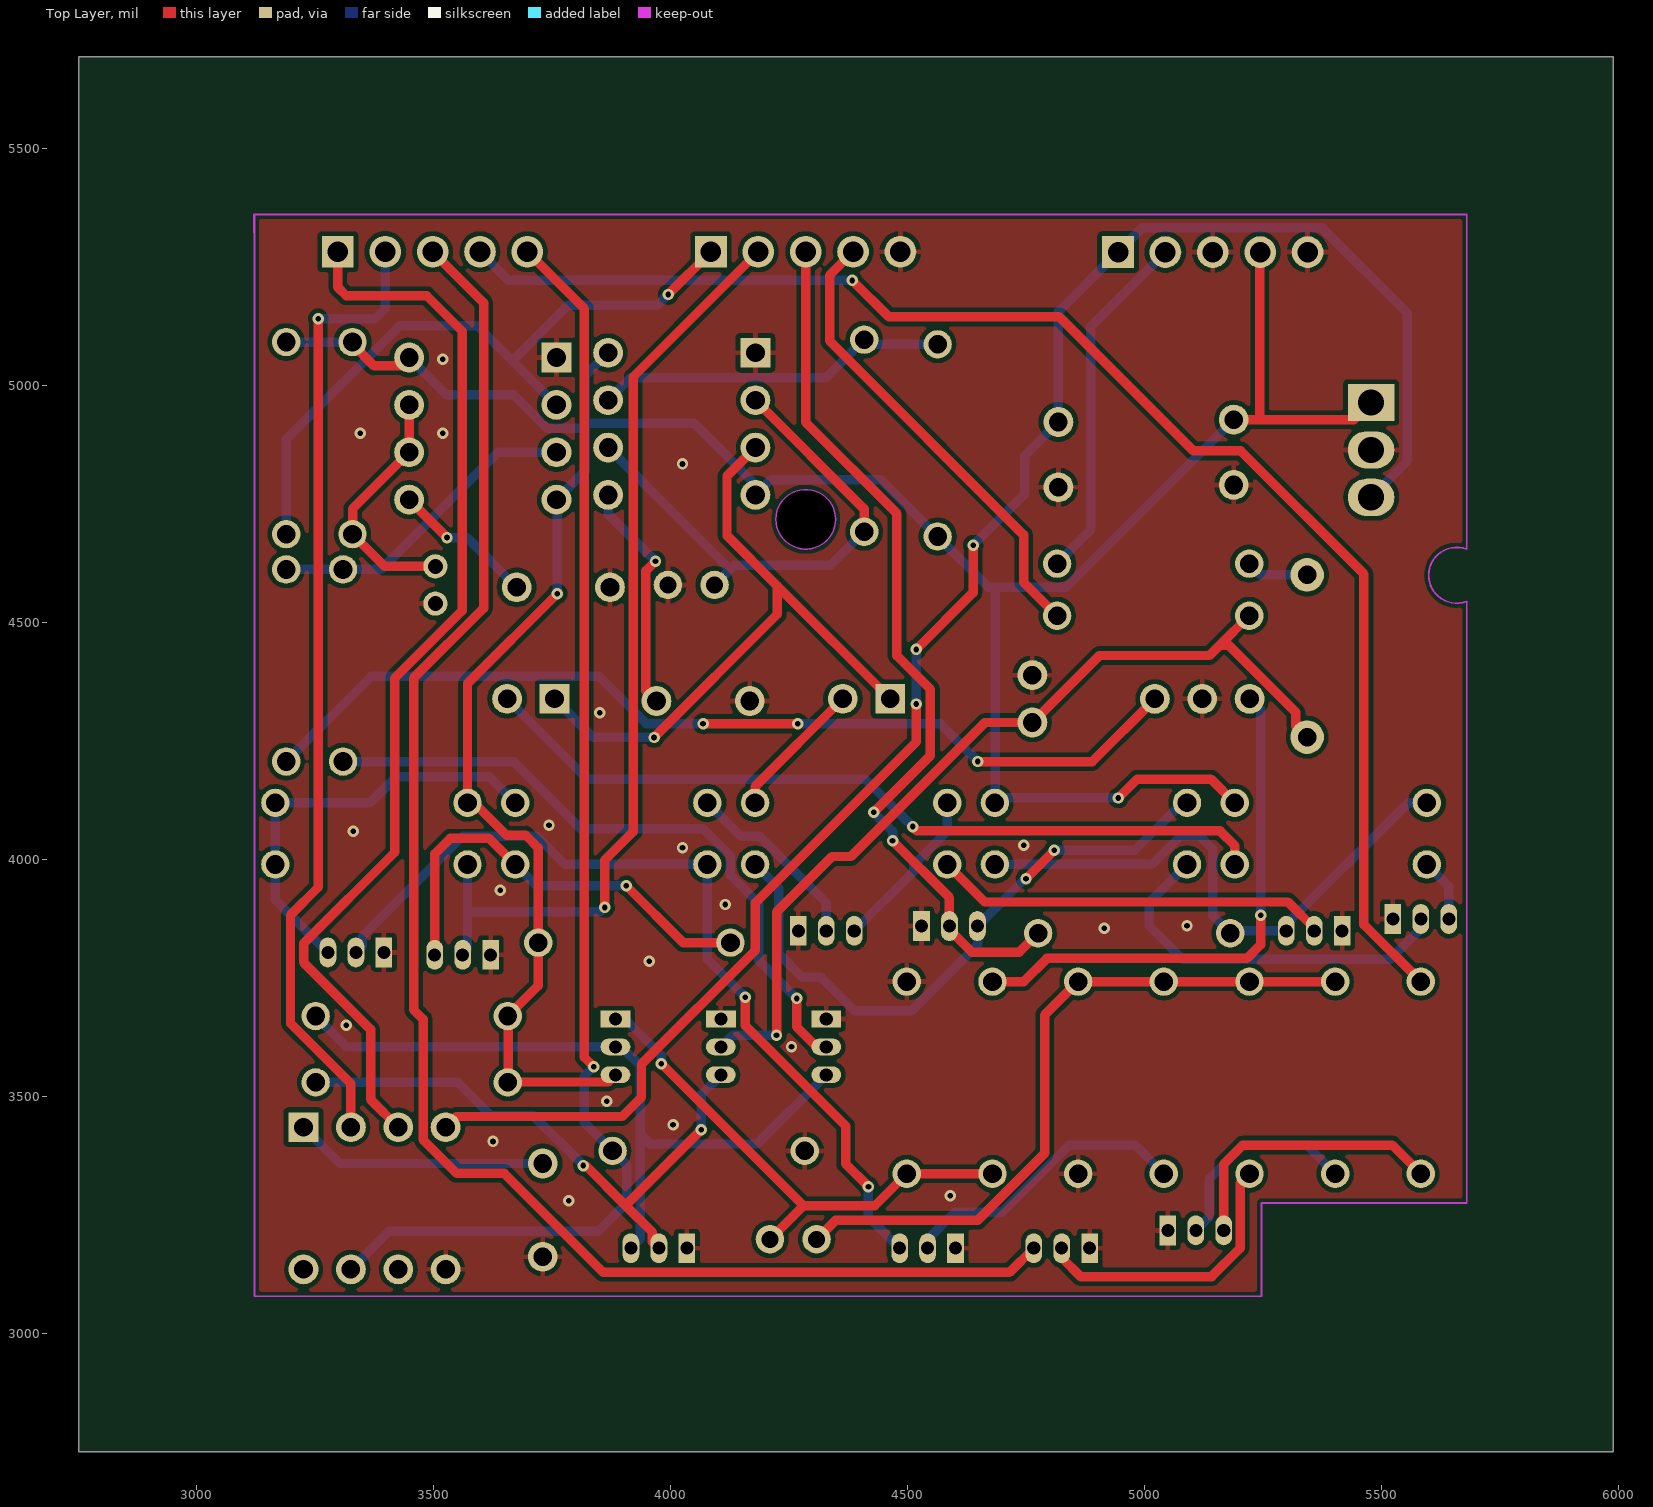
[diagram p0: Top Layer view]
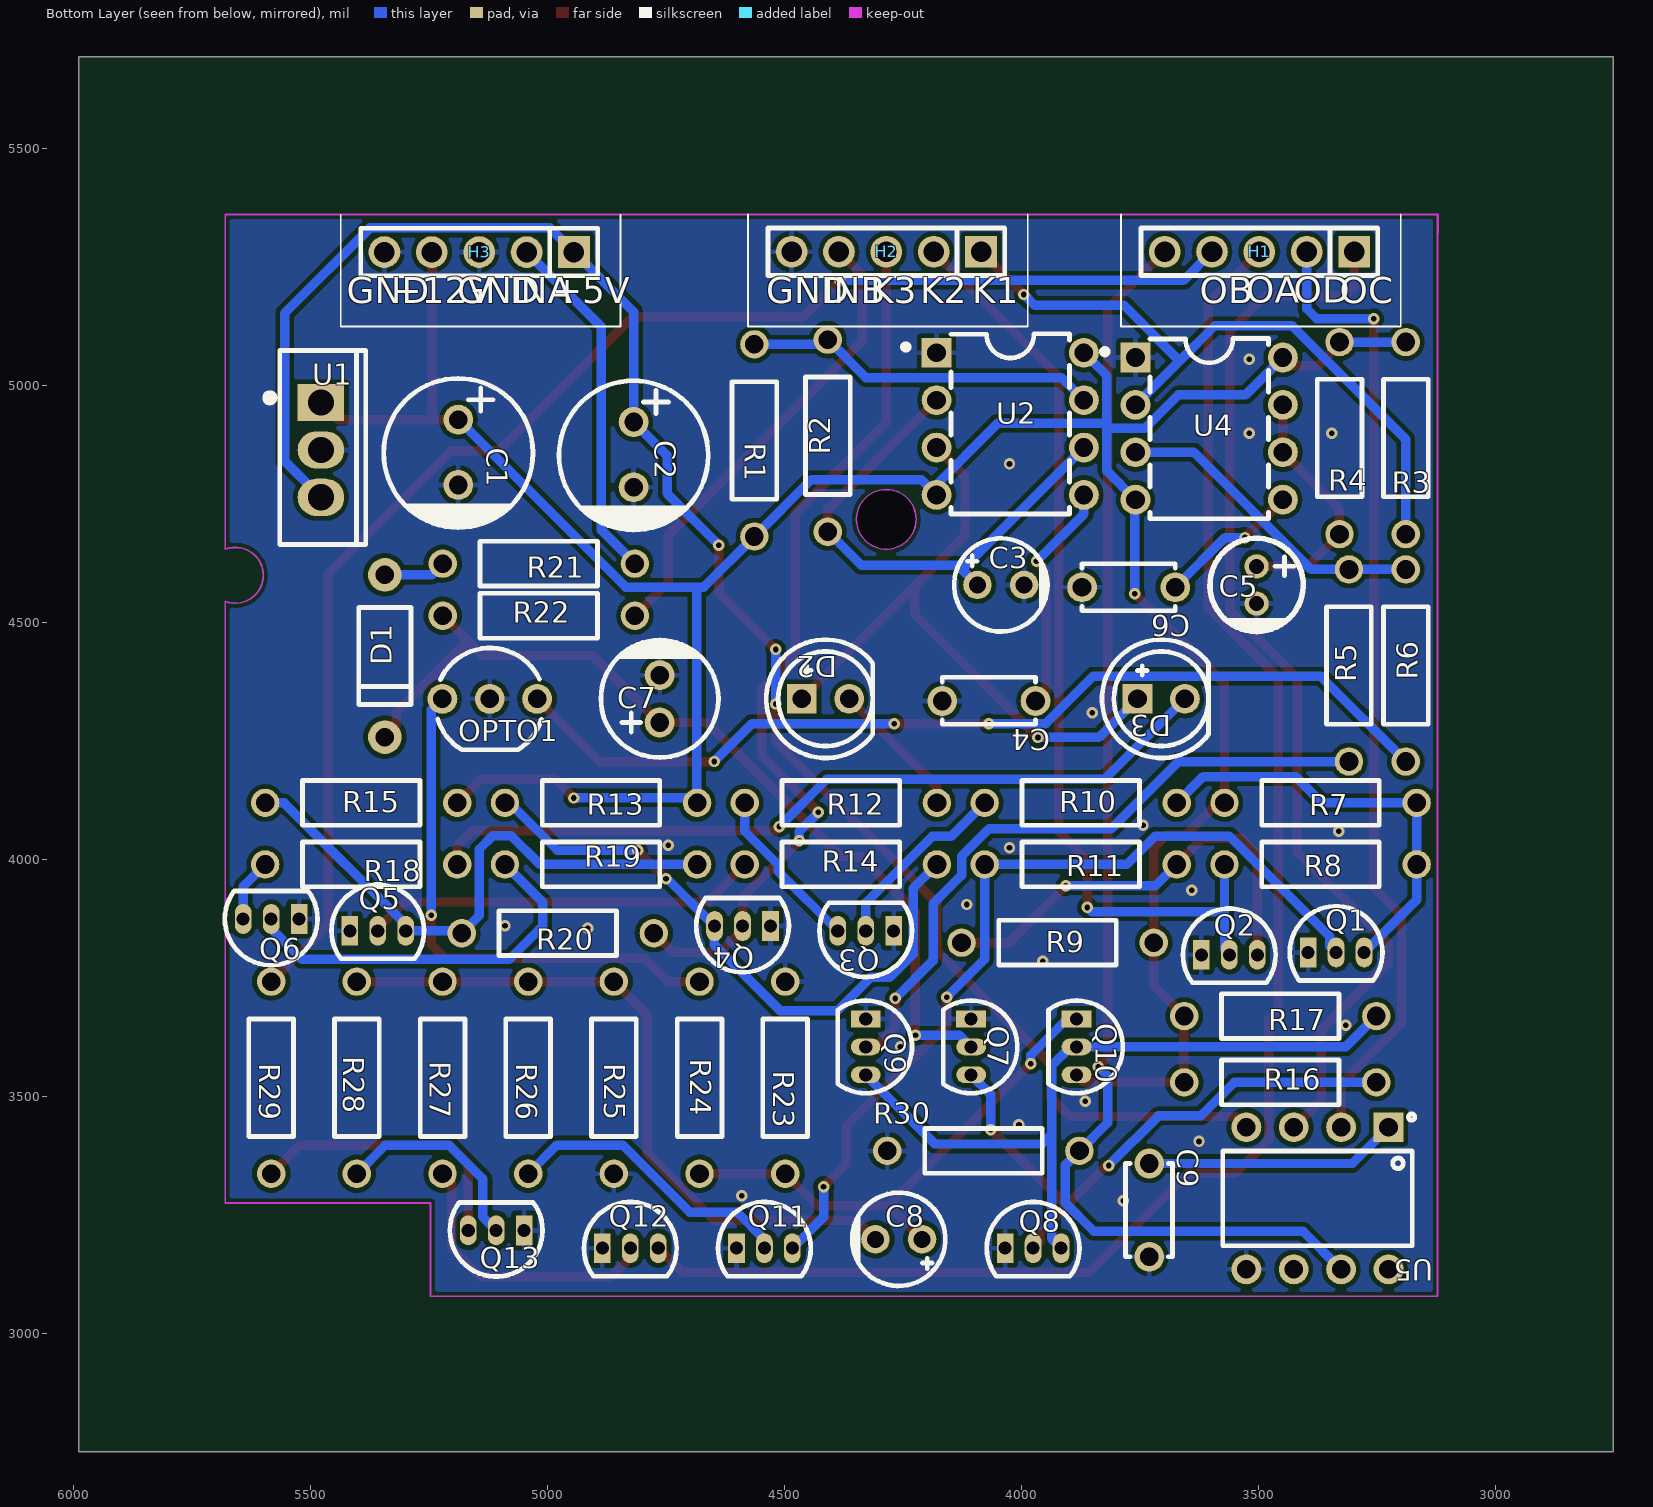
[diagram p1: Bottom Layer view, seen from below]
# Altium PCB MISC89097.pcbdoc
Units mil, origin at the board's own origin, x right, y up, seen from the top; angles counter-clockwise.
Board outline 3240 x 2945 mil, 2 copper layers (Top Layer, Bottom Layer), stack 62.206 mil thick; 63 components, 46 nets, 168 pads, 51 vias.

## Layer stack, top to bottom
Top Solder Mask Layer: solder mask 0.394, Dk 3.3
Top Layer: signal copper 1.379
Dielectric1: surface 59.449, FR4, Dk 4.5
Bottom Layer: signal copper 1.378
Bottom Solder Mask Layer: solder mask 0.394, Dk 3.3

## Board outline
5990,2750 2750,2750 2750,5695 5990,5695
cut-out: 4347.99,4718.11 cw(c4285,4718.11) 4222.01,4718.11 cw(c4285,4718.11)

## Design rules (kind name [scope] priority, off if disabled: settings)
BoardOutlineClearance copperThickness2oz_1 [All] p2 off: genericclearance=8 ignorepadtopadclearanceinfootprint=FALSE except(0: Arc-SplitContinuation Track-SplitContinuation SMDPad-SplitContinuation THPad-SplitContinuation Via-SplitContinuation Fill-SplitContinuation Region-SplitContinuation Poly-SplitContinuation Text-SplitContinuation Hole-SplitContinuation; 6: Arc-CutoutEdge Track-CutoutEdge SMDPad-CutoutEdge THPad-CutoutEdge Via-CutoutEdge Text-CutoutEdge; 6.9: Hole-OutlineEdge Hole-CutoutEdge; 10: Poly-OutlineEdge Poly-CutoutEdge; 11.8: Arc-OutlineEdge Track-OutlineEdge SMDPad-OutlineEdge THPad-OutlineEdge Via-OutlineEdge Fill-OutlineEdge Region-OutlineEdge Text-OutlineEdge Fill-CutoutEdge Region-CutoutEdge)
BoardOutlineClearance Plane_innerPlane_1 [All] p4 off: genericclearance=4 ignorepadtopadclearanceinfootprint=FALSE except(0: Arc-SplitContinuation Track-SplitContinuation SMDPad-SplitContinuation THPad-SplitContinuation Via-SplitContinuation Fill-SplitContinuation Region-SplitContinuation Poly-SplitContinuation Text-SplitContinuation Hole-SplitContinuation; 6: Arc-CutoutEdge Track-CutoutEdge SMDPad-CutoutEdge THPad-CutoutEdge Via-CutoutEdge Text-CutoutEdge; 6.9: Hole-OutlineEdge Hole-CutoutEdge; 10: Poly-OutlineEdge Poly-CutoutEdge; 11.8: Arc-OutlineEdge Track-OutlineEdge SMDPad-OutlineEdge THPad-OutlineEdge Via-OutlineEdge Fill-OutlineEdge Region-OutlineEdge Text-OutlineEdge Fill-CutoutEdge Region-CutoutEdge)
BoardOutlineClearance Copper_copperRegion_1 [All] p6 off: genericclearance=4 ignorepadtopadclearanceinfootprint=FALSE except(0: Arc-SplitContinuation Track-SplitContinuation SMDPad-SplitContinuation THPad-SplitContinuation Via-SplitContinuation Fill-SplitContinuation Region-SplitContinuation Poly-SplitContinuation Text-SplitContinuation Hole-SplitContinuation; 6: Arc-CutoutEdge Track-CutoutEdge SMDPad-CutoutEdge THPad-CutoutEdge Via-CutoutEdge Text-CutoutEdge; 6.9: Hole-OutlineEdge Hole-CutoutEdge; 10: Poly-OutlineEdge Poly-CutoutEdge; 11.8: Arc-OutlineEdge Track-OutlineEdge SMDPad-OutlineEdge THPad-OutlineEdge Via-OutlineEdge Fill-OutlineEdge Region-OutlineEdge Text-OutlineEdge Fill-CutoutEdge Region-CutoutEdge)
BoardOutlineClearance copperThickness1oz_1 [All] p8: genericclearance=4 ignorepadtopadclearanceinfootprint=FALSE except(0: Arc-SplitContinuation Track-SplitContinuation SMDPad-SplitContinuation THPad-SplitContinuation Via-SplitContinuation Fill-SplitContinuation Region-SplitContinuation Poly-SplitContinuation Text-SplitContinuation Hole-SplitContinuation; 6: Arc-CutoutEdge Track-CutoutEdge SMDPad-CutoutEdge THPad-CutoutEdge Via-CutoutEdge Text-CutoutEdge; 6.9: Hole-OutlineEdge Hole-CutoutEdge; 10: Poly-OutlineEdge Poly-CutoutEdge; 11.8: Arc-OutlineEdge Track-OutlineEdge SMDPad-OutlineEdge THPad-OutlineEdge Via-OutlineEdge Fill-OutlineEdge Region-OutlineEdge Text-OutlineEdge Fill-CutoutEdge Region-CutoutEdge)
Clearance copperThickness2oz [All] p1 off: gap=8 ignorepadtopadclearanceinfootprint=FALSE except(6: SMDPad-Track SMDPad-SMDPad THPad-Track SMDPad-THPad THPad-THPad Track-Via SMDPad-Via THPad-Via Via-Via Fill-SMDPad Region-SMDPad Fill-THPad Region-THPad Fill-Via Region-Via Fill-Fill Fill-Region Region-Region Arc-Track Arc-SMDPad Arc-THPad Arc-Via Fill-Arc Region-Arc Arc-Arc Text-Track SMDPad-Text Text-THPad Text-Via Fill-Text Region-Text Arc-Text Text-Text; 6.9: Hole-Track Hole-SMDPad Hole-THPad Hole-Via Fill-Hole Region-Hole Hole-Arc Hole-Text; 10: Poly-Track Poly-SMDPad Poly-THPad Poly-Via Poly-Fill Poly-Region Poly-Poly Poly-Arc Poly-Text Poly-Hole; 11.8: Fill-Track Region-Track)
Clearance Plane_innerPlane [All] p3 off: gap=4 ignorepadtopadclearanceinfootprint=FALSE except(6: SMDPad-Track SMDPad-SMDPad THPad-Track SMDPad-THPad THPad-THPad Track-Via SMDPad-Via THPad-Via Via-Via Fill-SMDPad Region-SMDPad Fill-THPad Region-THPad Fill-Via Region-Via Fill-Fill Fill-Region Region-Region Arc-Track Arc-SMDPad Arc-THPad Arc-Via Fill-Arc Region-Arc Arc-Arc Text-Track SMDPad-Text Text-THPad Text-Via Fill-Text Region-Text Arc-Text Text-Text; 6.9: Hole-Track Hole-SMDPad Hole-THPad Hole-Via Fill-Hole Region-Hole Hole-Arc Hole-Text; 10: Poly-Track Poly-SMDPad Poly-THPad Poly-Via Poly-Fill Poly-Region Poly-Poly Poly-Arc Poly-Text Poly-Hole; 11.8: Fill-Track Region-Track)
Clearance Copper_copperRegion [All] p5 off: gap=4 ignorepadtopadclearanceinfootprint=FALSE except(6: SMDPad-Track SMDPad-SMDPad THPad-Track SMDPad-THPad THPad-THPad Track-Via SMDPad-Via THPad-Via Via-Via Fill-SMDPad Region-SMDPad Fill-THPad Region-THPad Fill-Via Region-Via Fill-Fill Fill-Region Region-Region Arc-Track Arc-SMDPad Arc-THPad Arc-Via Fill-Arc Region-Arc Arc-Arc Text-Track SMDPad-Text Text-THPad Text-Via Fill-Text Region-Text Arc-Text Text-Text; 6.9: Hole-Track Hole-SMDPad Hole-THPad Hole-Via Fill-Hole Region-Hole Hole-Arc Hole-Text; 10: Poly-Track Poly-SMDPad Poly-THPad Poly-Via Poly-Fill Poly-Region Poly-Poly Poly-Arc Poly-Text Poly-Hole; 11.8: Fill-Track Region-Track)
Clearance copperThickness1oz [All] p7: gap=4 ignorepadtopadclearanceinfootprint=FALSE except(6: SMDPad-Track SMDPad-SMDPad THPad-Track SMDPad-THPad THPad-THPad Track-Via SMDPad-Via THPad-Via Via-Via Fill-SMDPad Region-SMDPad Fill-THPad Region-THPad Fill-Via Region-Via Fill-Fill Fill-Region Region-Region Arc-Track Arc-SMDPad Arc-THPad Arc-Via Fill-Arc Region-Arc Arc-Arc Text-Track SMDPad-Text Text-THPad Text-Via Fill-Text Region-Text Arc-Text Text-Text; 6.9: Hole-Track Hole-SMDPad Hole-THPad Hole-Via Fill-Hole Region-Hole Hole-Arc Hole-Text; 10: Poly-Track Poly-SMDPad Poly-THPad Poly-Via Poly-Fill Poly-Region Poly-Poly Poly-Arc Poly-Text Poly-Hole; 11.8: Fill-Track Region-Track)
DiffPairsRouting differentialPair [All] p1: maxlimit=6 minlimit=6 mostfreqgap=6 toplayer_minwidth=5 toplayer_prefwidth=10 toplayer_maxwidth=100 toplayer_mingap=6 toplayer_prefgap=6 toplayer_maxgap=6 bottomlayer_minwidth=5 bottomlayer_prefwidth=10 bottomlayer_maxwidth=100 bottomlayer_mingap=6 bottomlayer_prefgap=6 bottomlayer_maxgap=6 maxuncoupledlength=10
HoleToHoleClearance otherClearance [All] p1: gap=11.8 allowstackedmicrovias=TRUE
Length netLength [All] p1: minlimit=0 maxlimit=0
PasteMaskExpansion pasteMaskExpansion [All] p1: expansion=0
PlaneConnect innerPlane [All] p1: planeconnectstyle=Relief reliefexpansion=20 reliefentries=4 reliefconductorwidth=10 reliefairgap=10
PolygonConnect copperRegion [All] p1: connectstyle=Relief reliefconductorwidth=10 reliefentries=4 polygonreliefangle="90 Angle" airgapwidth=10 via.connectstyle=Relief via.reliefconductorwidth=10 via.reliefentries=4 via.polygonreliefangle="90 Angle" via.airgapwidth=10
RoutingVias viaSize [All] p1: holewidth=12 width=24 viastyle="Through Hole" minholewidth=11.8 minwidth=19.7 maxholewidth=248 maxwidth=393.7
SolderMaskExpansion solderMaskExpansion [IsVia] p1: expansion=-1000 istentingtop=TRUE
SolderMaskExpansion solderMaskExpansion [All] p2: expansion=2 istentingtop=FALSE
Width copperThickness2oz_2 [All] p1 off: maxlimit=100 minlimit=8 preferedwidth=10
Width copperThickness1oz_2 [All] p2: maxlimit=100 minlimit=5 preferedwidth=20

## Components (designator, comment, footprint, x,y, rotation, side; value= is the part's Value field where it differs from the comment)
C1 "100uF" CAP-TH_BD8.0-P3.50-D0.6-FD_1 5188.33,4859.58 r270 bottom
C2 "100uF" CAP-TH_BD8.0-P3.50-D0.6-FD_1 4818.33,4854.58 r270 bottom
C3 "22uF" CAP-TH_BD5.0-P2.5-D0.5-FD 4043.33,4579.58 r180 bottom
C4 "100nF" CAP-TH_L5.0-W2.5-P5.00-D1.0 4068.33,4334.58 r0 bottom
C5 "100UF" CAP-TH_BD5.0-P2.00-D0.8-FD 3503.33,4579.58 r270 bottom
C6 "100nF" CAP-TH_L5.0-W2.5-P5.00-D1.0 3773.33,4574.58 r0 bottom
C7 "4.7uF" CAP-TH_BD6.3-P2.50-D1.0-FD 4763.33,4339.24 r90 bottom
C8 "22uF" CAP-TH_BD5.0-P2.5-D0.5-FD 4258.65,3198.4 r0 bottom
C9 "100nF" CAP-TH_L5.0-W2.5-P5.00-D1.0 3730,3260 r270 bottom
D1 "" DO_1N4007 5343.33,4429.58 r90 bottom
D2 "" LED-TH_5mm 4413.3,4339.24 r180 bottom
D3 "" LED-TH_5mm 3704.64,4339.24 r180 bottom
H1 "" HDR-TH_5P-P2.54-V-M 3497.46,5282.81 r0 bottom
H2 "" HDR-TH_5P-P2.54-V-M 4284.86,5282.81 r0 bottom
H3 "" HDR-TH_5P-P2.54-V-M 5144.19,5282.23 r0 bottom
OPTO1 "38K infrared receiver, side-mounted" OPTO-TH_3P-BD5.9-P2.54 5121.96,4339.11 r270 bottom
Q1 "9013G" TO-92-3_L4.9-W3.7-P1.27-L 3335.46,3803.92 r180 bottom
Q2 "9013G" TO-92-3_L4.9-W3.7-P1.27-L 3560.94,3798.92 r180 bottom
Q3 "9013G" TO-92-3_L4.9-W3.7-P1.27-L 4328.33,3849.58 r0 bottom
Q4 "9013G" TO-92-3_L4.9-W3.7-P1.27-L 4588.33,3859.58 r0 bottom
Q5 "9013G" TO-92-3_L4.9-W3.7-P1.27-L 5358.33,3849.58 r180 bottom
Q6 "9013G" TO-92-3_L4.9-W3.7-P1.27-L 5583.33,3874.58 r0 bottom
Q7 "9013G" TO-92-3_L4.9-W3.7-P1.27-L 4105.83,3604.58 r270 bottom
Q8 "9013G" TO-92-3_L4.9-W3.7-P1.27-L 3975,3179.58 r180 bottom
Q9 "9013G" TO-92-3_L4.9-W3.7-P1.27-L 4328.33,3604.58 r270 bottom
Q10 "9013G" TO-92-3_L4.9-W3.7-P1.27-L 3883.33,3604.58 r270 bottom
Q11 "9013G" TO-92-3_L4.9-W3.7-P1.27-L 4542.3,3179.58 r180 bottom
Q12 "9013G" TO-92-3_L4.9-W3.7-P1.27-L 4825.32,3179.58 r180 bottom
Q13 "9013G" TO-92-3_L4.9-W3.7-P1.27-L 5108.33,3217.22 r0 bottom
R1 "10kΩ" Res_1/4W 4563.33,4884.58 r270 bottom
R2 "68kΩ" Res_1/4W 4408.33,4894.58 r90 bottom
R3 "20kΩ" Res_1/4W 3188.33,4889.58 r90 bottom
R4 "680kΩ" Res_1/4W 3328.33,4889.58 r90 bottom
R5 "27kΩ" Res_1/4W 3308.33,4409.58 r90 bottom
R6 "5.1kΩ" Res_1/4W 3188.33,4409.58 r90 bottom
R7 "10kΩ" Res_1/4W 3368.33,4119.58 r0 bottom
R8 "51kΩ" Res_1/4W 3368.33,3989.58 r180 bottom
R9 "5.1kΩ" Res_1/4W 3923.33,3824.58 r180 bottom
R10 "51kΩ" Res_1/4W 3874.58,4119.58 r180 bottom
R11 "51kΩ" Res_1/4W 3874.58,3989.58 r180 bottom
R12 "5.1kΩ" Res_1/4W 4380.83,4119.58 r180 bottom
R13 "10kΩ" Res_1/4W 4887.08,4119.58 r180 bottom
R14 "51kΩ" Res_1/4W 4380.83,3989.58 r180 bottom
R15 "10kΩ" Res_1/4W 5393.33,4119.58 r180 bottom
R16 "51kΩ" Res_1/4W 3453.33,3529.58 r180 bottom
R17 "5.1kΩ" Res_1/4W 3453.33,3669.58 r180 bottom
R18 "10kΩ" Res_1/4W 5393.33,3989.58 r180 bottom
R19 "51kΩ" Res_1/4W 4887.08,3989.58 r180 bottom
R20 "51kΩ" Res_1/4W 4978.33,3844.58 r0 bottom
R21 "100Ω" Res_1/4W 5018.33,4624.58 r180 bottom
R22 "5.1kΩ" Res_1/4W 5018.33,4514.58 r180 bottom
R23 "20kΩ" Res_1/4W 4498.33,3539.58 r90 bottom
R24 "27kΩ" Res_1/4W 4679.16,3539.58 r270 bottom
R25 "20kΩ" Res_1/4W 4860,3539.58 r270 bottom
R26 "2kΩ" Res_1/4W 5040.83,3539.58 r270 bottom
R27 "2kΩ" Res_1/4W 5221.66,3539.58 r270 bottom
R28 "27kΩ" Res_1/4W 5402.5,3539.58 r270 bottom
R29 "300Ω" Res_1/4W 5583.33,3539.58 r270 bottom
R30 "20kΩ" Res_1/4W 4080,3385 r180 bottom
U1 "L7805" TO-220AB-3_L10.4-W4.6-P2.54-L 5478.33,4864.58 r270 bottom
U2 "NE555" PDIP-8_L9.6-W6.4-P2.54-LS7.9-BL-1 4023.33,4919.58 r270 bottom
U4 "NE555" PDIP-8_L9.6-W6.4-P2.54-LS7.9-BL-1 3603.33,4909.58 r270 bottom
U5 "" DIP-8_L9.9-W6.4-P2.54-LS7.6-BL 3375,3285 r0 bottom

## Footprints (in the part's own frame and the unit in brackets; to place one, negate y for a bottom-side part, rotate by r counter-clockwise, add the part's x,y. Pads: shape width x height; smd on the part's side, far side on the other; paste and mask are expansions set on the pad)
CAP-TH_BD5.0-P2.00-D0.8-FD [mm]
  round 1.3 hole 0.8: 1(-1,0) 2(1,0)
  silkscreen extent -2.5,-2.5 2.5,2.5
CAP-TH_BD5.0-P2.5-D0.5-FD [mil]
  round 60 hole 36: 1(-49.21,0) 2(49.21,0)
  silkscreen extent -98,-98 98,98
CAP-TH_BD6.3-P2.50-D1.0-FD [mm]
  round 1.6 hole 1: 1(-1.27,0) 2(1.27,0)
  silkscreen extent -3.15,-3.15 3.17,3.15
CAP-TH_BD8.0-P3.50-D0.6-FD_1 [mm]
  round 1.6 hole 1: 1(-1.75,0) 2(1.75,0)
  silkscreen extent -3.96,-4 4.04,4
CAP-TH_L5.0-W2.5-P5.00-D1.0 [mm]
  round 1.6 hole 1: 1(-2.5,0) 2(2.5,0)
  silkscreen extent -2.5,-1.27 2.5,1.25
DIP-8_L9.9-W6.4-P2.54-LS7.6-BL [mil]
  rect 63x63 hole 39.37: 1(-150,-150.01)
  round 63 hole 39.37: 2(-50,-150.01) 3(50,-150.01) 4(150,-150.01) 5(150,149.99) 6(50,149.99) 7(-50,149.99) 8(-150,149.99)
  silkscreen extent -206,-178 200,100
DO_1N4007 [mm]
  round 1.8 hole 1 paste+0 mask+0.051: 1(-4.35,0) 2(4.35,0)
  silkscreen extent -2.6,-1.4 2.6,1.4
HDR-TH_5P-P2.54-V-M [mm]
  rect 1.7x1.7 hole 1.1: 1(-5.08,0)
  round 1.7 hole 1.1: 2(-2.54,0) 3(0,0) 4(2.54,0) 5(5.08,0)
  silkscreen extent -6.35,-1.27 6.35,1.27
LED-TH_5mm [mm]
  rect 1.6x1.6 hole 1 paste+0 mask+0.051: 1(-1.27,0)
  round 1.6 hole 1 paste+0 mask+0.051: 2(1.27,0)
  silkscreen extent -3.17,-3.17 2.54,3.17
OPTO-TH_3P-BD5.9-P2.54 [mm]
  round 1.6 hole 1: 1(0,2.54) 2(0,0) 3(0,-2.54)
  silkscreen extent -2.73,-2.79 2.72,2.77
PDIP-8_L9.6-W6.4-P2.54-LS7.9-BL-1 [mil]
  rect 63x63 hole 39.37: 1(-150,-155.51)
  round 63 hole 39.37: 2(-50,-155.51) 3(50,-155.51) 4(150,-155.51) 5(150,155.5) 6(50,155.5) 7(-50,155.5) 8(-150,155.5)
  silkscreen extent -190,-226 190,125
Res_1/4W [mil]
  round 60 hole 39.37 paste+0 mask+2: 1(-202.76,0) 2(202.76,0)
  silkscreen extent -124,-47 124,47
TO-92-3_L4.9-W3.7-P1.27-L [mm]
  rect 0.9x1.6 hole 0.7: 1(-1.5,0)
  oval 0.9x1.6 hole 0.7: 2(0,0) 3(1.5,0)
  silkscreen extent -2.48,-1.5 2.48,2.48
TO-220AB-3_L10.4-W4.6-P2.54-L [mm]
  rect 2x2.5 hole 1.4: 1(-2.54,0)
  oval 2x2.5 hole 1.4: 2(0,0) 3(2.54,0)
  silkscreen extent -5.33,-2.94 5.08,2.4

## Via types
v1: diameter 24, hole 12, Top Layer to Bottom Layer, 29 vias
v2: diameter 24.02, hole 12, Top Layer to Bottom Layer, 22 vias

## Nets (pads, with @x,y where several pads share a name; then routed paths per layer and width w, separated by ;. In a path a pad name is that pad's centre, name@x,y a point inside that pad or via, vN(x,y) a via of type N, cw(c..) or ccw(c..) an arc to the next point about the centre after c; other vN are vias at no path point)
$1N1448: R1.1 R2.2 U2.7 | length 752.6
  Bottom Layer w20: U2.7 3915.58,5017.34 4328.33,5017.34 R2.2 4418.33,5087.34 R1.1
$1N1530: C3.1 R2.1 U2.2 U2.6 | length 1100.1
  Top Layer w20: U2.2 4408.33,4740.09 R2.1
  Bottom Layer w20: U2.6 4123.36,4614.04 4127,4614.04 ; C3.1 4127,4614.04 ; R2.1 4337.62,4621.11 4134.07,4621.11 4127,4614.04
$1N1865: C5.1 R4.1 U4.6 U4.7 | length 525.8
  Top Layer w20: R4.1 R4.1@3329.03,4686.13 ; U4.7 U4.6 3329.03,4740.79 R4.1@3329.03,4686.13 ; C5.1 3396.2,4618.95 R4.1@3329.03,4686.13
$1N2164: C6.1 U4.5 | length 303.7
  Top Layer w20: U4.5 v1(3527.82,4679.58)
  Bottom Layer w20: v1(3527.82,4679.58) 3569.91,4679.58 C6.1
$1N2217: R5.2 R6.2 U4.3 | length 672.9
  Bottom Layer w20: R6.2 R5.2 3388.33,4612.34 3635.57,4859.58 U4.3
$1N2360: Q1.3 R7.1 R8.2 R10.2 | length 913.7
  Bottom Layer w20: Q1.3 3165.57,3914.75 R8.2 R7.1 3365.57,4119.58 3420.99,4175 3616.4,4175 R10.2
$1N2559: Q2.3 R9.1 R11.2 | length 942.2
  Top Layer w20: Q2.3 3501.88,4011.88 3535,4045 3616.4,4045 R11.2 ; v1(3906.09,3944.58) 4026.09,3824.58 R9.1
  Bottom Layer w20: R11.2 3716.82,3944.58 v1(3906.09,3944.58)
$1N2623: Q3.3 R12.1 | length 351.3
  Bottom Layer w20: Q3.3 4512.88,3975.08 4512.88,3988.87 4583.59,4059.58 R12.1
$1N2687: Q4.3 R13.1 R14.2 | length 1327.7
  Top Layer w20: v1(4749.84,3959.58) v1(4809.84,4019.58)
  Bottom Layer w20: R14.2 4228.39,3939.26 4228.39,3800.59 4277.68,3751.3 4317.68,3751.3 4388.39,3680.59 4508.39,3680.59 4648.39,3820.59 Q4.3@4648.39,3860.59 ; Q4.3 Q4.3@4648.39,3860.59 ; v1(4749.84,3959.58) 4747.39,3959.58 Q4.3@4648.39,3860.59 ; v1(4809.84,4019.58) 4979.58,4019.58 5079.58,4119.58 R13.1
$1N2751: Q5.3 R15.1 R19.2 R20.2 | length 1225.6
  Bottom Layer w20: R19.2 5016.09,3989.58 5076.51,4050 5115.86,4050 5144.14,4021.72 5144.14,3881.53 R20.2 5186.09,3849.58 Q5.3 5299.28,3862.77 5556.09,4119.58 R15.1
$1N2815: Q6.3 R18.1 | length 134.2
  Bottom Layer w20: R18.1 5642.39,3943.29 Q6.3
$1N2904: D2.2 R12.2 | length 296.4
  Top Layer w20: R12.2 4178.07,4154.02 D2.2
$1N2951: D3.2 R18.2 | length 1704.1
  Top Layer w20: v1(4510.57,4069.58) 4519.86,4060.29 5159.71,4060.29 5190.57,4029.43 R18.2
  Bottom Layer w20: D3.2 3824.3,4169.58 4410.57,4169.58 v1(4510.57,4069.58)
$1N3054: Q3.2 R10.1 | length 397.4
  Bottom Layer w20: R10.1 4148.05,4048.87 4188.05,4048.87 4328.33,3908.59 Q3.2
$1N3795: Q5.2 R14.1 | length 835.8
  Top Layer w20: R14.1 4662.83,3910.34 5302.83,3910.34 5358.33,3854.84 Q5.2
$1N3920: Q6.2 R19.1 | length 812.2
  Bottom Layer w20: R19.1 5009.84,3909.58 5009.84,3860.16 5080.42,3789.58 5518.33,3789.58 5583.33,3854.58 Q6.2
$1N4638: OPTO1.1 R6.1 | length 2037.5
  Top Layer w20: v1(4068.33,4286.82) v1(4268.33,4286.82) ; v1(4648.33,4206.82) 4889.66,4206.82 OPTO1.1
  Bottom Layer w20: R6.1 3368.33,4386.82 3848.33,4386.82 3948.33,4286.82 v1(4068.33,4286.82) ; v1(4268.33,4286.82) 4568.33,4286.82 v1(4648.33,4206.82)
$1N4740: D1.2 R21.1 | length 132.1
  Bottom Layer w20: R21.1 5244.83,4600.84 D1.2
$1N4912: C7.1 D1.1 Q7.2 R22.1 | length 1926.4
  Top Layer w20: v1(4223.33,3629.24) 4223.33,3889.24 4340.49,4006.4 4380.49,4006.4 4663.33,4289.24 C7.1 4904.75,4430.67 5137.18,4430.67 5158.39,4451.88 ; R22.1 5158.39,4451.88 ; D1.1 5319.81,4281.84 5319.81,4310.46 5178.39,4451.88 5158.39,4451.88
  Bottom Layer w20: Q7.2 4130.49,3629.24 v1(4223.33,3629.24)
$1N4955: Q7.3 Q8.2 R16.2 | length 1240.1
  Top Layer w20: v1(3815.57,3354.01) 3820.57,3354.01 3904.71,3269.87 ; Q8.2 3961.28,3193.3 3961.28,3213.3 3904.71,3269.87 ; v1(4064.71,3429.87) 3904.71,3269.87
  Bottom Layer w20: R16.2 3550.42,3529.58 3621.13,3458.87 3710.71,3458.87 v1(3815.57,3354.01) ; v1(4064.71,3429.87) 4064.71,3504.41 Q7.3
$1N5034: Q8.3 Q9.3 Q10.2 R17.2 | length 1583.3
  Bottom Layer w20: R17.2 3315.57,3604.58 Q10.2 3895.94,3604.58 3935.94,3564.58 3935.94,3419.58 ; Q8.3 3935.94,3199.58 3935.94,3419.58 ; Q9.3 4182.39,3399.58 3955.94,3399.58 3935.94,3419.58
$1N5190: C8.1 Q10.1 R23.1 R24.2 | length 1097.7
  Top Layer w20: v1(3980.15,3569.11) 4280.15,3269.11 ; C8.1 4280.15,3269.11 ; R24.2 R23.1 4430.62,3269.11 4280.15,3269.11
  Bottom Layer w20: Q10.1 3889.44,3657.53 3909.44,3657.53 3980.15,3586.82 v1(3980.15,3569.11)
$1N5220: Q9.2 R5.1 | length 1398.3
  Top Layer w20: v1(4266.09,3706.82) 4266.09,3646.82 4308.33,3604.58 Q9.2
  Bottom Layer w20: R5.1 3668.33,4206.82 3809.75,4065.4 4067.51,4065.4 4126.09,4006.82 4126.09,3966.82 4186.09,3906.82 4186.09,3786.82 v1(4266.09,3706.82)
$1N5329: OPTO1.3 R24.1 | length 1126.8
  Top Layer w20: R24.1 4745.19,3742.34 4794.19,3791.35 5216.35,3791.35 5245.19,3820.18 v1(5245.19,3882.34)
  Bottom Layer w20: OPTO1.3 5245.19,4315.89 v1(5245.19,3882.34)
$1N5364: C8.2 R25.1 R26.1 R27.1 R28.1 | length 1490.9
  Top Layer w20: C8.2 4347.86,3238.4 4647.86,3238.4 4789.28,3379.82 4789.28,3671.62 R25.1 R26.1 R27.1 R28.1
$1N5425: Q11.2 R26.2 | length 624.3
  Bottom Layer w20: Q11.2 4542.3,3198.29 4599.41,3255.4 4699.41,3255.4 4840.83,3396.82 4980.83,3396.82 R26.2
$1N5516: Q12.2 R27.2 | length 603.3
  Top Layer w20: Q12.2 4825.32,3159.58 4865.32,3119.58 5141.66,3119.58 5201.66,3179.58 5201.66,3316.82 R27.2
$1N5612: Q13.2 R28.2 | length 440.3
  Bottom Layer w20: Q13.2 5137.22,3246.11 5137.22,3326.11 5207.93,3396.82 5342.5,3396.82 R28.2
$1N5640: Q13.3 R29.2 | length 597.2
  Top Layer w20: Q13.3 5167.39,3357.22 5206.99,3396.82 5523.33,3396.82 R29.2
$1N7574: C4.1 U2.5 | length 493.9
  Top Layer w20: v1(3967.82,4629.58) 3947.82,4609.58 3947.82,4356.67 C4.1
  Bottom Layer w20: U2.5 3867.82,4729.58 v1(3967.82,4629.58)
$1N8703: D2.1 D3.1 U2.3 | length 1369.6
  Top Layer w20: v1(3964.91,4257.64) 4224.91,4517.64 4224.91,4577.64 ; U2.3 4118.84,4809.58 4118.84,4683.7 4224.91,4577.64 ; D2.1 4224.91,4577.64
  Bottom Layer w20: D3.1 3836.25,4257.64 v1(3964.91,4257.64)
$1N9904: C9.1 U5.1 | length 536.7
  Bottom Layer w20: U5.1 3301.58,3358.43 C9.1
$1N10142: Q1.2 Q11.3 R11.1 | length 1858.3
  Top Layer w20: v1(4157.34,3709.58) 4157.34,3649.58 4369.47,3437.45 4369.47,3357.45 v1(4417.34,3309.58)
  Bottom Layer w20: Q1.2 3348.99,3817.45 3348.99,3837.45 3561.12,4049.58 3717.34,4049.58 3777.34,3989.58 R11.1 4077.34,3789.58 v1(4157.34,3709.58) ; v1(4417.34,3309.58) 4417.34,3245.48 Q11.3
+5V: C2.1 H3.1 U1.3 U5.4 | length 3766.7
  Top Layer w20: U5.4 3547.62,3457.62 3897.62,3457.62 3938.33,3498.33 3938.33,3568.33 4178.33,3808.33 4178.33,3908.33 4518.33,4248.33 v1(4518.33,4328.33) ; v1(4518.33,4443.48) 4638.33,4563.48 v1(4638.33,4663.48)
  Bottom Layer w20: v1(4518.33,4328.33) v1(4518.33,4443.48) ; v1(4638.33,4663.48) 4747.62,4772.77 4747.62,4852.77 C2.1 4818.33,5156.36 H3.1 4995,5333.04 5375,5333.04 5555,5153.04 5555,4841.25 U1.3
+12V: C1.1 H3.4 Q10.3 R1.2 R3.2 R4.2 R7.2 R9.2 R13.2 R15.2 R16.1 R17.1 U1.1 U2.4 U2.8 U4.4 U4.8 | length 6098.6
  Top Layer w20: R4.2 3329.15,5091.53 3329.15,5086.53 3373.79,5041.88 3430.12,5041.88 U4.8 ; R7.2 R7.2@3571.09,4121.83 ; R16.1 3656.93,3530.42 R16.1@3656.93,3550.42 ; R17.1 R17.1@3656.93,3670.42 ; v1(3760.37,4561.11) 3571.09,4371.83 R7.2@3571.09,4121.83 ; Q10.3 3868.23,3530.42 3676.93,3530.42 R16.1@3656.93,3550.42 ; v1(4944.78,4129.93) 4984.78,4169.93 5140.22,4169.93 R15.2 ; C1.1 5243.33,4928.48 ; H3.4 5243.33,5281.36 5243.33,4928.48 ; U1.1 5442.23,4928.48 5243.33,4928.48 ; R7.2@3571.09,4121.83 3582.81,4121.83 3653.52,4051.12 3693.88,4051.12 3720.57,4024.43 R9.2 3720.57,3734.06 R17.1@3656.93,3670.42 ; R16.1@3656.93,3550.42 R17.1@3656.93,3670.42
  Bottom Layer w20: R3.2 R4.2 ; U4.8 3526.69,4980.71 3668.55,4980.71 3739.26,4910 3815,4910 ; U4.4 U4.4@3760.37,4761.11 ; v1(3760.37,4561.11) U4.4@3760.37,4761.11 ; U2.8 3819.26,5021.02 3819.26,4919.26 ; U2.4 U2.4@4189.87,4780.61 ; R13.2 4684.78,4120.04 R13.2@4684.78,4129.93 ; v1(4944.78,4129.93) R13.2@4684.78,4129.93 ; C1.1 4834.78,4574.93 4684.78,4574.93 ; U4.4@3760.37,4761.11 3819.26,4820 3819.26,4919.26 ; 3819.26,4919.26 3820.61,4920.61 4049.87,4920.61 U2.4@4189.87,4780.61 ; U2.4@4189.87,4780.61 4211.08,4801.82 4443.33,4801.82 R1.2 4670.22,4574.93 4684.78,4574.93 ; R13.2@4684.78,4129.93 4684.78,4574.93
GND: C1.2 C2.2 C3.2 C4.2 C5.2 C6.2 C7.2 C9.2 H2.5 H3.3 H3.5 OPTO1.2 Q1.1 Q2.1 Q3.1 Q4.1 Q5.1 Q6.1 Q7.1 Q8.1 Q9.1 Q11.1 Q12.1 Q13.1 R23.2 R25.2 R30.1 U1.2 U2.1 U4.1 U5.5
  other v2: 3785,3280 4590,3290 3625,3405 4005,3440 3865,3490 4254.87,3604.58 3315,3650 3955,3785 4915,3855 5089.69,3860.16 4115,3905 3640,3935 4025,4025 4745,4030 3330,4060 3743.17,4072.34 3850,4310 4025,4835 3345,4900 3518.66,4900 3518.66,5056.09
INA: H3.2 R21.2 | length 752.3
  Bottom Layer w20: R21.2 4886.28,4695.29 4886.28,5124.31 H3.2
INB: H2.4 R22.2 | length 987.5
  Top Layer w20: H2.4 4335.57,5233.52 4335.57,5094.58 4744.86,4685.29 4744.86,4585.29 R22.2
INC: H1.5 R30.2 U5.7 | length 2750.9
  Top Layer w20: H1.5 3817.46,5162.81 3817.46,3582.81 v1(3837.46,3562.81)
  Bottom Layer w20: U5.7 3405.28,3215.28 3846.96,3215.28 3906.96,3275.28 3906.96,3355.28 R30.2 3817.46,3444.78 3817.46,3542.81 v1(3837.46,3562.81)
K1: H2.1 R3.1 U4.2 | length 1453.6
  Top Layer w20: v1(3994.63,5192.57) H2.1
  Bottom Layer w20: R3.1 3188.33,4886.82 3428.33,5126.82 3591.6,5126.82 3665.85,5052.57 ; U4.2 3665.85,5052.57 ; v1(3994.63,5192.57) 3972.05,5170 3783.27,5170 3665.85,5052.57
K2: H2.2 Q2.2 R8.1 | length 2041
  Top Layer w20: v1(3860.94,3898.92) 3860.94,3998.92 3920.94,4058.92 3920.94,5018.88 H2.2
  Bottom Layer w20: R8.1 3571.09,3889.63 ; v1(3860.94,3898.92) 3851.65,3889.63 3571.09,3889.63 ; 3571.09,3829.07 3571.09,3809.07 Q2.2 3560.94,3818.92 3571.09,3829.07 ; 3571.09,3829.07 3571.09,3889.63
K3: H2.3 Q4.2 R20.1 | length 1879.5
  Top Layer w20: H2.3 4284.86,4923.05 4477.62,4730.29 4477.62,4430.29 4548.33,4359.58 4548.33,4219.58 v1(4428.33,4099.58) ; v1(4468.33,4039.58) 4588.33,3919.58 Q4.2 4588.33,3851.82 4635.57,3804.58 4735.57,3804.58 R20.1
  Bottom Layer w20: v1(4428.33,4099.58) 4468.33,4059.58 v1(4468.33,4039.58)
OUTA: H1.3 Q12.3 | length 3414.4
  Top Layer w20: H1.3 3605,5175.27 3605,4530.35 3457.46,4382.81 3457.46,3682.81 3477.46,3662.81 3477.46,3408.38 3548.17,3337.67 3648.17,3337.67 3857.46,3128.38 4715.06,3128.38 Q12.3
OUTB: H1.4 R29.1 | length 3057.4
  Top Layer w20: v1(4383.33,5222.34) 4460.49,5145.18 4820.49,5145.18 5103.33,4862.34 5203.33,4862.34 5463.33,4602.34 5463.33,3862.34 R29.1
  Bottom Layer w20: H1.4 3657.93,5222.34 v1(4383.33,5222.34)
OUTC: H1.1 U5.3 | length 2277.7
  Top Layer w20: H1.1 3297.46,5207.54 3315,5190 3485,5190 3560,5115 3560,4525.35 3417.46,4382.81 3417.46,4015.26 3225.01,3822.81 3225.01,3782.81 3366.43,3641.39 3366.43,3493.58 U5.3
OUTD: H1.2 U5.2 | length 2054
  Top Layer w20: v2(3256.04,5141.39) 3256.04,3941.39 3197.46,3882.81 3197.46,3654.31 3325.01,3526.77 U5.2
  Bottom Layer w20: v2(3256.04,5141.39) 3376.39,5141.39 3397.46,5162.46 H1.2
pads on no net: U5.6 U5.8

## Polygon pours and split planes (outlines as drawn)
GND on Bottom Layer (solid, remove dead copper, pour order 2): 3050,5405 3050,3025 5740,3025 5740,5405
GND on Top Layer (solid, remove dead copper, pour order 0): 3000,5445 3000,3000 5740,3000 5740,5445

## Keep-outs
Board Outline Layer:
  region: 4347.99,4718.11 cw(c4285,4718.11) 4222.01,4718.11 cw(c4285,4718.11)
  circle w0.1: c4285,4718.11 r62.99
  region: 4347.99,4718.11 4347.6,4711.06 4346.41,4704.09 4344.46,4697.31 4341.75,4690.78 4338.34,4684.6 4334.25,4678.84 4329.54,4673.57 4324.27,4668.86 4318.51,4664.77 4312.33,4661.36 4305.8,4658.65 4299.02,4656.7 4292.05,4655.51 4285,4655.12 4277.95,4655.51 4270.98,4656.7 4264.2,4658.65 4257.67,4661.36 4251.49,4664.77 4245.73,4668.86 4240.46,4673.57 4235.75,4678.84 4231.66,4684.6 4228.25,4690.78 4225.54,4697.31 4223.59,4704.09 4222.4,4711.06 4222.01,4718.11 4222.4,4725.16 4223.59,4732.13 4225.54,4738.92 4228.25,4745.44 4231.66,4751.62 4235.75,4757.39 4240.46,4762.65 4245.73,4767.36 4251.49,4771.45 4257.67,4774.86 4264.2,4777.57 4270.98,4779.52 4277.95,4780.71 4285,4781.1 4292.05,4780.71 4299.02,4779.52 4305.8,4777.57 4312.33,4774.86 4318.51,4771.45 4324.27,4767.36 4329.54,4762.65 4334.25,4757.39 4338.34,4751.62 4341.75,4745.44 4344.46,4738.92 4346.41,4732.13 4347.6,4725.16
  lines w3.94: 3121.05,5282.81 3120.3,5361.55 5680.33,5361.55 5680.33,4655.05 ccw(c5658.96,4600) 5680.33,4544.95 5680.33,3274.94 5247.26,3274.94 5247.26,3078.09 3121.28,3078.09 3121.28,5361.55

## Silkscreen, mask and mechanical layers (free items; w line width, h text height)
Bottom Silkscreen Layer:
  lines w3.94: 3199.04,5361.55 3199.04,5125.33 3789.59,5125.33 3789.59,5361.55 ; 3986.44,5361.55 3986.44,5125.33 4576.99,5125.33 4576.99,5361.55 ; 4845.77,5360.97 4845.77,5124.75 5436.32,5124.75 5436.32,5360.97
  text "OC" at 3328.33,5174.58 h55.12
  text "OD" at 3425,5175 h55.12
  text "OA" at 3525,5175 h55.12
  text "OB" at 3623.33,5174.58 h55.12
  text "K1" at 4103.33,5174.58 h55.12
  text "K2" at 4213.33,5174.58 h55.12
  text "K3" at 4318.33,5174.58 h55.12
  text "INB" at 4418.33,5174.58 h55.12
  text "GND" at 4538.33,5174.58 h55.12
  text "INA" at 5078.33,5174.58 h55.12
  text "+12V" at 5328.33,5174.58 h55.12
  text "GND" at 5423.33,5174.58 h55.12
  text "+5V" at 4990.06,5174 h55.12
  text "GND" at 5190.06,5174 h55.12
Mechanical Layer:
  circle w0.1: c4285,4718.11 r62.99